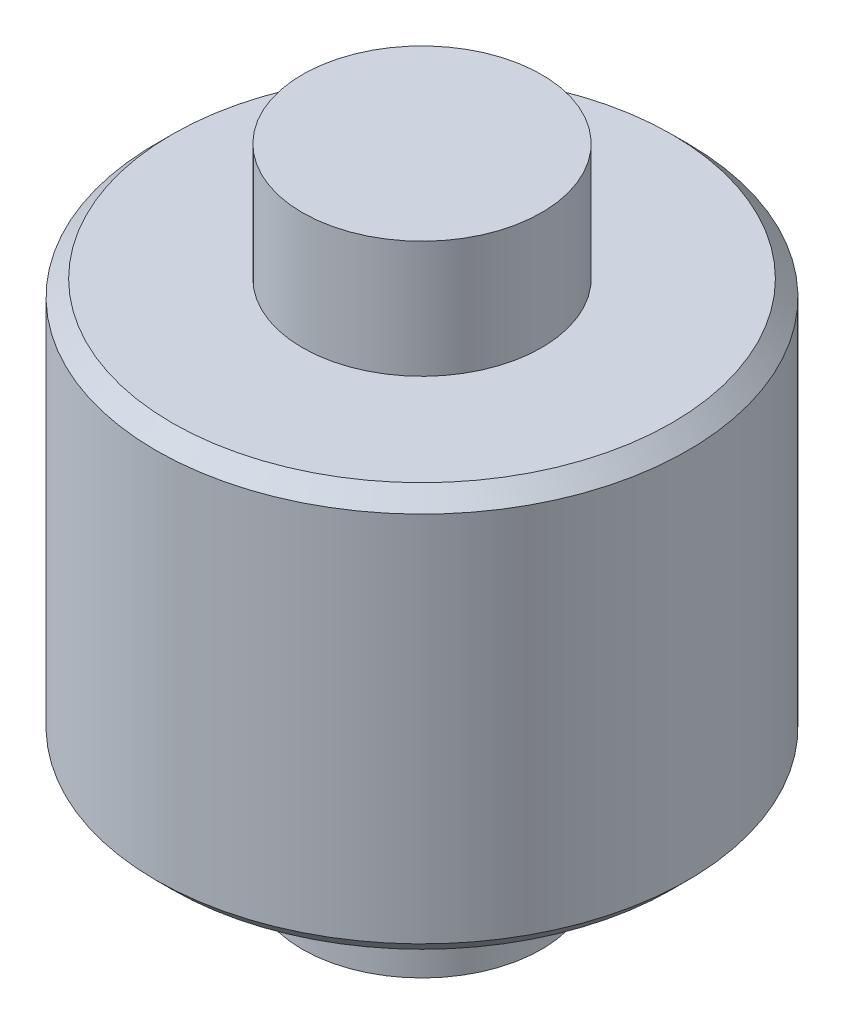
from build123d import *

# Parameters (mm, degrees)
SKETCH1_R                = 45
BOSS_EXTRUDE1_DEPTH      = 240
BOSS_EXTRUDE2_DEPTH      = 76
BOSS_EXTRUDE2_DEPTH_BACK = 76
SKETCH2_R                = 100
CHAMFER1_SIZE            = 6


with BuildPart() as part:
    # Sketch1 → Boss-Extrude1 (new body)
    with BuildSketch(Plane(origin=(0, 0, 0), x_dir=(1, 0, 0), z_dir=(0, 1, 0))):
        with Locations(Location((0, 0, 0), (0, 0, 270))):
            Circle(SKETCH1_R)
    extrude(amount=BOSS_EXTRUDE1_DEPTH)

    # Sketch2 → Boss-Extrude2 (add, two sides: drawn at the far end of the back side and taken through both)
    with BuildSketch(Plane(origin=(0, 120, 0), x_dir=(1, 0, 0), z_dir=(0, 1, 0)).offset(-BOSS_EXTRUDE2_DEPTH_BACK)):
        with Locations(Location((0, 0, 0), (0, 0, 270))):
            Circle(SKETCH2_R)
    extrude(amount=BOSS_EXTRUDE2_DEPTH + BOSS_EXTRUDE2_DEPTH_BACK)

    # Chamfer1
    chamfer1_edges = [part.edges().sort_by_distance(p)[0] for p in [
        (0, 44, -100),
        (0, 196, -100),
    ]]
    chamfer(chamfer1_edges, length=CHAMFER1_SIZE)


solid = part.part
